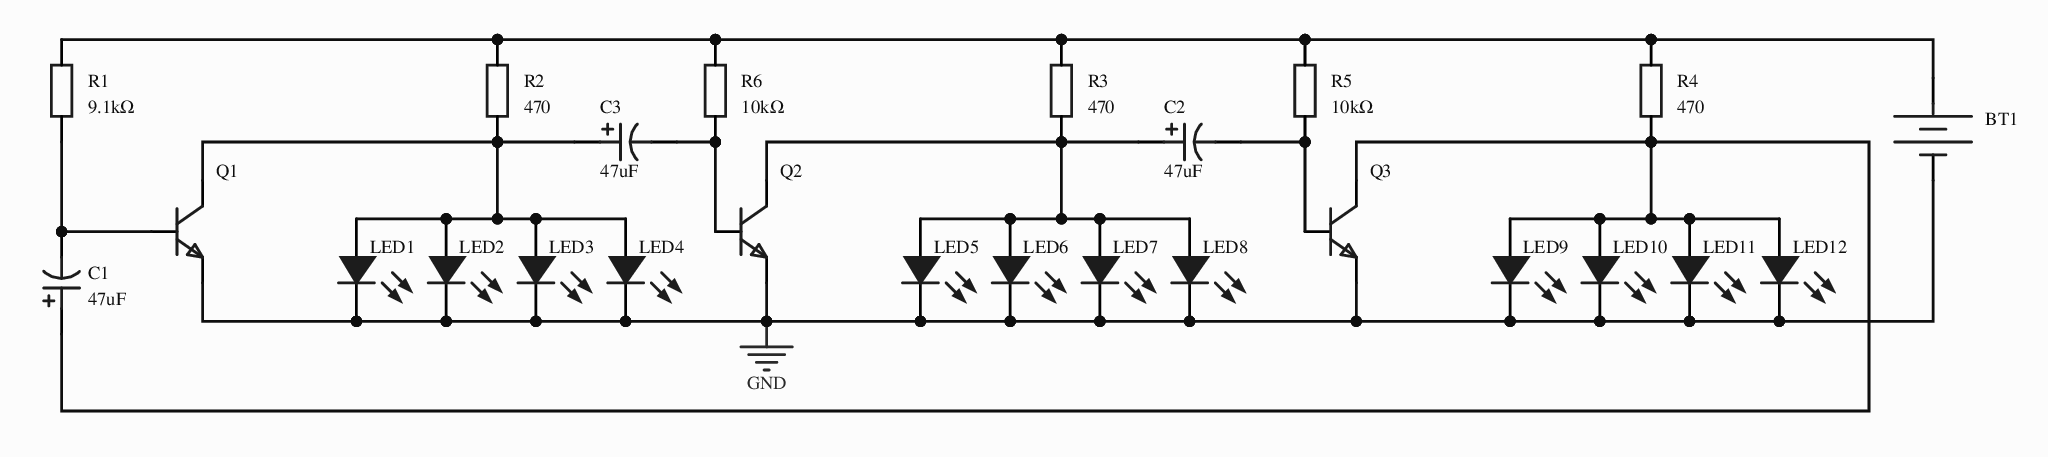
[diagram p0: MISC75405-3.schdoc]
# Altium project MISC75405-2.PrjPcb
1 sheet, 25 parts. Net scope: global (net labels, ports and power ports of the same name join across sheets).
Board file: MISC75405.pcbdoc

## Sheet MISC75405-3.schdoc
size 297 x 209 mm; Version: V1.0; @Project Name: MISC75405; @Update Date: 2026-04-13; @Create Date: 2026-04-13; @Board Name: MISC75405; @Create Time: 10:13:34; @Page Count: 1; @Page No: 1; @Schematic Name: MISC75405; @Update Time: 10:13:34; Size: A4

### Parts
BT1  9V battery wire clip Cu 100mm  [BAT-TH_2P-9VBATTERY]  (value not drawn)
C1  47uF  [CAP-TH_BD6.3-P2.50-D0.5-FD]
C2  47uF  [CAP-TH_BD6.3-P2.50-D0.5-FD]
C3  47uF  [CAP-TH_BD6.3-P2.50-D0.5-FD]
LED1  (no value)  [LED-TH_5mm]
LED2  (no value)  [LED-TH_5mm]
LED3  (no value)  [LED-TH_5mm]
LED4  (no value)  [LED-TH_5mm]
LED5  (no value)  [LED-TH_5mm]
LED6  (no value)  [LED-TH_5mm]
LED7  (no value)  [LED-TH_5mm]
LED8  (no value)  [LED-TH_5mm]
LED9  (no value)  [LED-TH_5mm]
LED10  (no value)  [LED-TH_5mm]
LED11  (no value)  [LED-TH_5mm]
LED12  (no value)  [LED-TH_5mm]
Q1  (no value)  [S8050_TO_92]
Q2  (no value)  [S8050_TO_92]
Q3  (no value)  [S8050_TO_92]
R1  9.1kΩ  [Res_1/8W]
R2  470  [Res_1/8W]
R3  470  [Res_1/8W]
R4  470  [Res_1/8W]
R5  10kΩ  [Res_1/8W]
R6  10kΩ  [Res_1/8W]

### Nets
GND: BT1.2(-) LED1.2(A) LED2.2(A) LED3.2(A) LED4.2(A) LED5.2(A) LED6.2(A) LED7.2(A) LED8.2(A) LED9.2(A) LED10.2(A) LED11.2(A) LED12.2(A) Q1.1(E) Q2.1(E) Q3.1(E)
NetBT1_1: BT1.1(+) R1.2 R2.2 R3.2 R4.2 R5.2 R6.2
NetC1_1: C1.1 LED9.1(C) LED10.1(C) LED11.1(C) LED12.1(C) Q3.3(C) R4.1
NetC1_2: C1.2 Q1.2(B) R1.1
NetC2_1: C2.1 LED5.1(C) LED6.1(C) LED7.1(C) LED8.1(C) Q2.3(C) R3.1
NetC2_2: C2.2 Q3.2(B) R5.1
NetC3_1: C3.1 LED1.1(C) LED2.1(C) LED3.1(C) LED4.1(C) Q1.3(C) R2.1
NetC3_2: C3.2 Q2.2(B) R6.1

### Library data of the parts
BT1 = 9V电池铜线扣 铜100mm: 铜线扣; Manufacturer: QIJEY; AddInBom: yes; Contact coating: Nickel plating; Applicable battery specifications: 9V stacked battery; Symbol: 9V battery wire clip Cu 100MM; Device: 9V battery wire clip Cu 100mm; LCSC Part Name: 电池扣 9V电池铜线扣 铜100mm; SupplierPart: C70374; ManufacturerPart: 9V电池铜线扣 铜100mm; Supplier Footprint: -; JLCPCB Part Class: Extended Part; Datasheet: https://item.szlcsc.com/datasheet/9V%25E7%2594%25B5%25E6%25B1%25A0%25E9%2593%259C%25E7%25BA%25BF%25E6%2589%25A3%2520%25E9%2593%259C100mm/71469.html; Supplier: LCSC; ConvertToPcb: yes; FootprintName: BAT-TH_2P-9VBATTERY; Type: Battery clip
C1 = DHG016M476E110S1AA: 容值:47uF;精度:±20%;额定电压:16V;纹波电流:200mA@100kHz;等效串联电阻(ESR):570mΩ@100kHz;; Manufacturer: KNSCHA(科尼盛); AddInBom: yes; ModelId: 983aa343eddc42b59ebb10541a88166e0819f05c4eef4c71ace90d822a990e87; ModelTransform: 247.99486,248.229,0,90,0,0,0,0,-196.85; Tolerance: ±20%; Voltage Rating: 16V; Pin Spacing: 2.5mm; Lifetime: 2000hrs@105℃; Description: Capacitance 47uF; Tolerance ±20%; Rated voltage 16V; Ripple current 200mA@100kHz; ESR 570mΩ@100kHz;; Symbol: DHG016M476E110S1AA; Device: DHG016M476E110S1AA; LCSC Part Name: 47uF ±20% 16V; SupplierPart: C46550715; ManufacturerPart: DHG016M476E110S1AA; Supplier Footprint: 插件,D6.3xL11mm; Datasheet: https://item.szlcsc.com/datasheet/DHG016M476E110S1AA/48681555.html; Supplier: LCSC; ConvertToPcb: yes; FootprintName: CAP-TH_BD6.3-P2.50-D0.5-FD; ModelName: CAP-TH_BD6.3-P2.50-D0.5-FD; Value: 47uF; Ripple Current: 200mA@100kHz; Equivalent Series Resistance(ESR): 570mΩ@100kHz; Diameter: 6.3mm; Height - Seated (Max): 11mm; Operating Temperature: -40℃~+105℃
C2 C3 = DHG016M476E110S1AA: 容值:47uF;精度:±20%;额定电压:16V;纹波电流:200mA@100kHz;等效串联电阻(ESR):570mΩ@100kHz;; Manufacturer: KNSCHA(科尼盛); AddInBom: yes; ModelId: 983aa343eddc42b59ebb10541a88166e0819f05c4eef4c71ace90d822a990e87; ModelTransform: 247.99486,248.229,0,90,0,0,0,0,-196.85; Tolerance: ±20%; Voltage Rating: 16V; Pin Spacing: 2.5mm; Lifetime: 2000hrs@105℃; Symbol: DHG016M476E110S1AA; Device: DHG016M476E110S1AA; LCSC Part Name: 47uF ±20% 16V; SupplierPart: C46550715; ManufacturerPart: DHG016M476E110S1AA; Supplier Footprint: 插件,D6.3xL11mm; Datasheet: https://item.szlcsc.com/datasheet/DHG016M476E110S1AA/48681555.html; Supplier: LCSC; ConvertToPcb: yes; FootprintName: CAP-TH_BD6.3-P2.50-D0.5-FD; ModelName: CAP-TH_BD6.3-P2.50-D0.5-FD; Value: 47uF; Ripple Current: 200mA@100kHz; Equivalent Series Resistance(ESR): 570mΩ@100kHz; Diameter: 6.3mm; Height - Seated (Max): 11mm; Operating Temperature: -40℃~+105℃
LED1-LED12 = LED_TH-B_5mm: AddInBom: yes; ModelId: b0e300213b7e4bc9906214592eb37e0a0819f05c4eef4c71ace90d822a990e87; ModelName: LED-TH_BD5.0_Blue; ModelTransform: 177.89258,177.84487,480.30997,90,0,0,-1.9685,0,-389.76378; Symbol: LED_TH-B; Device: LED_TH-B_5mm; ConvertToPcb: yes; FootprintName: LED-TH_5mm; Supplier Footprint: 插件
Q1-Q3 = S8050_TO_NPN: ConvertToPcb: yes; ModelId: aafe8e06f2154e7c93506efd0d6632dd0819f05c4eef4c71ace90d822a990e87; ModelName: TO-92-3_L4.9-W3.7-P1.27-L; ModelTransform: 180.78,141.44,417.3,0,0,0,0,0,-200; Symbol: S8050_TO_NPN; Device: S8050_TO_NPN; AddInBom: yes; Supplier Footprint: TO-92; FootprintName: S8050_TO_92
R1-R6 = Res_AXIAL-1/8W: Symbol: Resistor; ConvertToPcb: yes; ModelId: b2b5ae7ae4c642178fe0039925c86a3f0819f05c4eef4c71ace90d822a990e87; ModelName: RES-TH_BD1.8-L3.2-P7.20-D0.4; ModelTransform: 282.86,66.88,253.09,0,0,0,0,0,-191; Device: Res_AXIAL-1/8W; AddInBom: yes; Supplier Footprint: 轴向引线; FootprintName: Res_1/8W
  R1: Value: 9.1kΩ
  R2-R4: Value: 470
  R5 R6: Value: 10kΩ